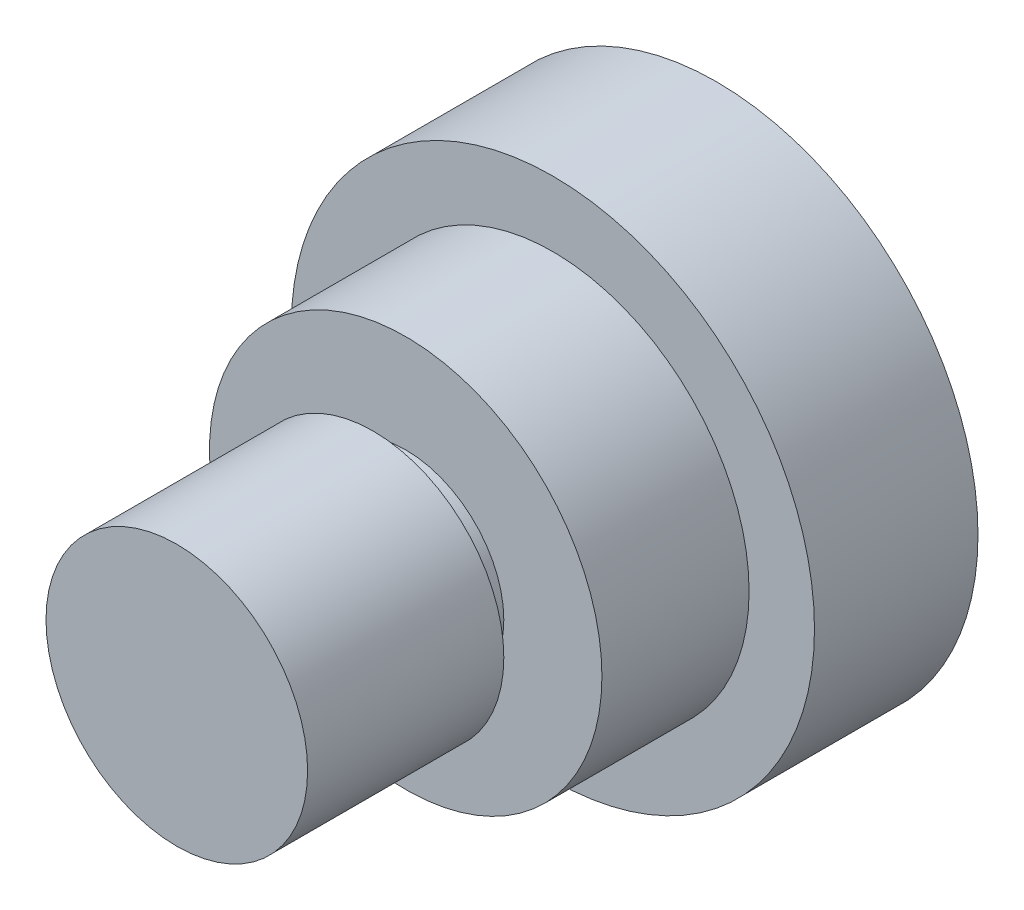
from build123d import *


with BuildPart() as part:
    # Sketch1 → Revolve1 (revolve)
    with BuildSketch(Plane(origin=(0, 0, 0), x_dir=(0, 0, -1), z_dir=(1, 0, 0)), mode=Mode.PRIVATE) as revolve1_sk:
        Polygon((16.5, 0), (16.5, 8), (11.5, 8), (11.5, 6), (7, 6), (7, 3), (6, 3), (6, 4), (0, 4), (0, 0), align=None)
    revolve(revolve1_sk.sketch.rotate(Axis((0, 0, 0), (0, 0, -1)), 90), axis=Axis((0, 0, 0), (0, 0, -1)))


solid = part.part
